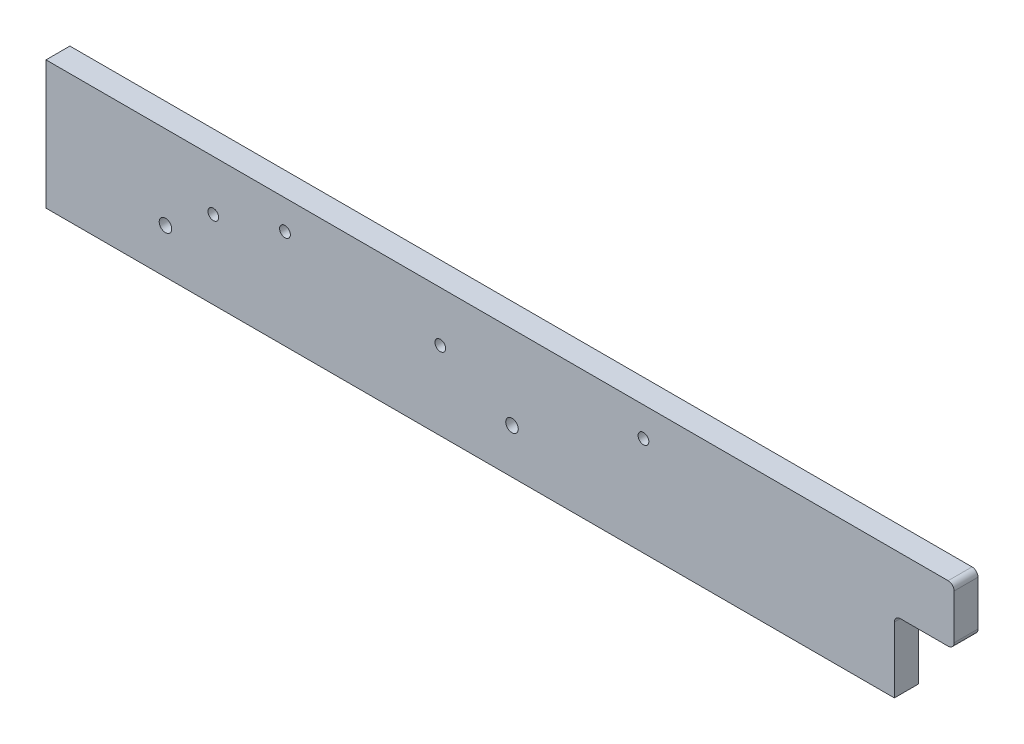
from build123d import *

# Parameters (mm, degrees)
SKETCH1_R                        = 9
BOSS_EXTRUDE1_DEPTH              = 40
M24_TAPPED_HOLE1_D               = 21
FILLET1_R                        = 10
SKETCH3_R                        = 9
SKETCH3_R_2                      = 9.680977079
BOSS_EXTRUDE2_DEPTH              = 25
M14_TAPPED_HOLE1_D               = 12
M14_TAPPED_HOLE1_DEPTH           = 40
M14_TAPPED_HOLE1_ON_FACE_2_D     = 12
M14_TAPPED_HOLE1_ON_FACE_2_DEPTH = 40


with BuildPart() as part:
    # Sketch1 → Boss-Extrude1 (new body)
    with BuildSketch(Plane.XY):
        Polygon((0, 215), (1520, 215), (1520, 120), (1420, 120), (1420, 0), (0, 0), align=None)
        with Locations((400, 166)):
            Circle(SKETCH1_R, mode=Mode.SUBTRACT)
        with Locations((280, 131)):
            Circle(SKETCH1_R, mode=Mode.SUBTRACT)
        with Locations((660, 131)):
            Circle(SKETCH1_R, mode=Mode.SUBTRACT)
        with Locations((1000, 166)):
            Circle(SKETCH1_R, mode=Mode.SUBTRACT)
    extrude(amount=BOSS_EXTRUDE1_DEPTH)

    # M24 Tapped Hole1 (through all)
    with Locations(Plane(origin=(780, 75, 40), x_dir=(1, 0, 0), z_dir=(0, 0, 1))):
        with Locations((0, 0), (-580, 0)):
            Hole(M24_TAPPED_HOLE1_D / 2)

    # Fillet1
    fillet1_edges = [part.edges().sort_by_distance(p)[0] for p in [
        (1520, 215, 20),
        (1520, 120, 20),
        (1420, 120, 20),
    ]]
    fillet(fillet1_edges, radius=FILLET1_R)

    # Sketch3 → Boss-Extrude2 (add)
    with BuildSketch(Plane(origin=(0, 0, 0), x_dir=(-1, 0, 0), z_dir=(0, 0, -1))):
        with Locations(Location((-1000, 166, 0), (0, 0, 90))):
            Circle(SKETCH3_R)
        with Locations((-400, 166)):
            Circle(SKETCH3_R_2)
    extrude(amount=-BOSS_EXTRUDE2_DEPTH)

    # M14 Tapped Hole1
    with Locations(Plane(origin=(1000, 166, 40), x_dir=(0, 1, 0), z_dir=(0, 0, 1))):
        with Locations((0, 0)):
            Hole(M14_TAPPED_HOLE1_D / 2, depth=M14_TAPPED_HOLE1_DEPTH)

    # M14 Tapped Hole1 on face 2
    with Locations(Plane(origin=(400, 166, 25), x_dir=(1, 0, 0), z_dir=(0, 0, 1))):
        with Locations((0, 0)):
            Hole(M14_TAPPED_HOLE1_ON_FACE_2_D / 2, depth=M14_TAPPED_HOLE1_ON_FACE_2_DEPTH)


solid = part.part
